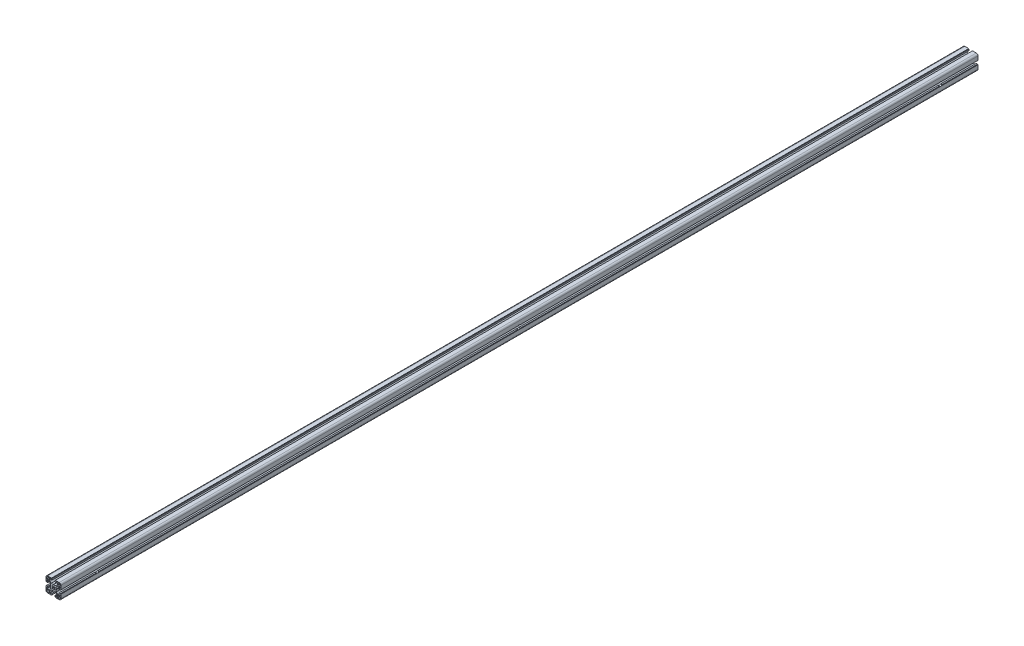
from build123d import *

# Parameters (mm, degrees)
EXTRUDE_1_DEPTH             = 2470
HOLE_WIZARD_2_D             = 6.6
HOLE_WIZARD_2_CBORE_D       = 11
HOLE_WIZARD_2_CBORE_DEPTH   = 6.8
HOLE_WIZARD_2_2_D           = 6.6
HOLE_WIZARD_2_2_CBORE_D     = 11
HOLE_WIZARD_2_2_CBORE_DEPTH = 6.8


with BuildPart() as part:
    # 草图1 → 凸台-拉伸1 (new body)
    with BuildSketch(Plane.XY):
        with BuildLine():
            Line((-18.9995, -4.100341675), (-18.9995, -5.100341675))
            Line((-18.9995, -5.100341675), (-19.9995, -5.100341675))
            Line((-19.9995, -5.100341675), (-19.9995, -15.500341675))
            ThreePointArc((-19.9995, -15.500341675), (-18.681480515, -18.682322191), (-15.4995, -20.000341675))
            Line((-15.4995, -20.000341675), (-5.0995, -20.000341675))
            Line((-5.0995, -20.000341675), (-5.0995, -19.000341675))
            Line((-5.0995, -19.000341675), (-4.0995, -19.000341675))
            Line((-4.0995, -19.000341675), (-4.0995, -15.500341675))
            Line((-4.0995, -15.500341675), (-6.5995, -15.500341675))
            Line((-6.5995, -15.500341675), (-6.5995, -16.500341675))
            ThreePointArc((-6.5995, -16.500341675), (-6.892393219, -17.207448457), (-7.5995, -17.500341675))
            Line((-7.5995, -17.500341675), (-9.7995, -17.500341675))
            ThreePointArc((-9.7995, -17.500341675), (-10.153053391, -17.353895066), (-10.2995, -17.000341675))
            Line((-10.2995, -17.000341675), (-10.2995, -11.997341675))
            Line((-10.2995, -11.997341675), (-5.9025, -7.600341675))
            Line((-5.9025, -7.600341675), (-0.5195, -7.600341675))
            Line((-0.5195, -7.600341675), (0.0005, -7.300341675))
            Line((0.0005, -7.300341675), (0.5195, -7.600341675))
            Line((0.5195, -7.600341675), (5.9035, -7.600341675))
            Line((5.9035, -7.600341675), (10.3005, -11.997341675))
            Line((10.3005, -11.997341675), (10.3005, -17.000341675))
            ThreePointArc((10.3005, -17.000341675), (10.154053391, -17.353895066), (9.8005, -17.500341675))
            Line((9.8005, -17.500341675), (7.6005, -17.500341675))
            ThreePointArc((7.6005, -17.500341675), (6.893393219, -17.207448457), (6.6005, -16.500341675))
            Line((6.6005, -16.500341675), (6.6005, -15.500341675))
            Line((6.6005, -15.500341675), (4.1005, -15.500341675))
            Line((4.1005, -15.500341675), (4.1005, -19.000341675))
            Line((4.1005, -19.000341675), (5.1005, -19.000341675))
            Line((5.1005, -19.000341675), (5.1005, -20.000341675))
            Line((5.1005, -20.000341675), (15.5005, -20.000341675))
            ThreePointArc((15.5005, -20.000341675), (18.682480515, -18.682322191), (20.0005, -15.500341675))
            Line((20.0005, -15.500341675), (20.0005, -5.100341675))
            Line((20.0005, -5.100341675), (19.0005, -5.100341675))
            Line((19.0005, -5.100341675), (19.0005, -4.100341675))
            Line((19.0005, -4.100341675), (15.5005, -4.100341675))
            Line((15.5005, -4.100341675), (15.5005, -6.600341675))
            Line((15.5005, -6.600341675), (16.5005, -6.600341675))
            ThreePointArc((16.5005, -6.600341675), (17.207606781, -6.893234894), (17.5005, -7.600341675))
            Line((17.5005, -7.600341675), (17.5005, -9.800341675))
            ThreePointArc((17.5005, -9.800341675), (17.354053391, -10.153895066), (17.0005, -10.300341675))
            Line((17.0005, -10.300341675), (11.9975, -10.300341675))
            Line((11.9975, -10.300341675), (7.6005, -5.903341675))
            Line((7.6005, -5.903341675), (7.6005, -0.520341675))
            Line((7.6005, -0.520341675), (7.3005, -0.000341675))
            Line((7.3005, -0.000341675), (7.6005, 0.519658325))
            Line((7.6005, 0.519658325), (7.6005, 5.902658325))
            Line((7.6005, 5.902658325), (11.9975, 10.299658325))
            Line((11.9975, 10.299658325), (17.0005, 10.299658325))
            ThreePointArc((17.0005, 10.299658325), (17.354053391, 10.153211715), (17.5005, 9.799658325))
            Line((17.5005, 9.799658325), (17.5005, 7.599658325))
            ThreePointArc((17.5005, 7.599658325), (17.207606781, 6.892551543), (16.5005, 6.599658325))
            Line((16.5005, 6.599658325), (15.5005, 6.599658325))
            Line((15.5005, 6.599658325), (15.5005, 4.099658325))
            Line((15.5005, 4.099658325), (19.0005, 4.099658325))
            Line((19.0005, 4.099658325), (19.0005, 5.099658325))
            Line((19.0005, 5.099658325), (20.0005, 5.099658325))
            Line((20.0005, 5.099658325), (20.0005, 15.499658325))
            ThreePointArc((20.0005, 15.499658325), (18.682480515, 18.68163884), (15.5005, 19.999658325))
            Line((15.5005, 19.999658325), (5.1005, 19.999658325))
            Line((5.1005, 19.999658325), (5.1005, 18.999658325))
            Line((5.1005, 18.999658325), (4.1005, 18.999658325))
            Line((4.1005, 18.999658325), (4.1005, 15.499658325))
            Line((4.1005, 15.499658325), (6.6005, 15.499658325))
            ThreePointArc((6.6005, 15.499658325), (6.393348977, 15.999658325), (6.6005, 16.499658325))
            ThreePointArc((6.6005, 16.499658325), (6.893393219, 17.206765106), (7.6005, 17.499658325))
            Line((7.6005, 17.499658325), (9.8005, 17.499658325))
            ThreePointArc((9.8005, 17.499658325), (10.154053391, 17.353211715), (10.3005, 16.999658325))
            Line((10.3005, 16.999658325), (10.3005, 11.996658325))
            Line((10.3005, 11.996658325), (5.9035, 7.599658325))
            Line((5.9035, 7.599658325), (0.5195, 7.599658325))
            Line((0.5195, 7.599658325), (0.0005, 7.299658325))
            Line((0.0005, 7.299658325), (-0.5195, 7.599658325))
            Line((-0.5195, 7.599658325), (-5.9025, 7.599658325))
            Line((-5.9025, 7.599658325), (-10.2995, 11.996658325))
            Line((-10.2995, 11.996658325), (-10.2995, 16.999658325))
            ThreePointArc((-10.2995, 16.999658325), (-10.153053391, 17.353211715), (-9.7995, 17.499658325))
            Line((-9.7995, 17.499658325), (-7.5995, 17.499658325))
            ThreePointArc((-7.5995, 17.499658325), (-6.892393219, 17.206765106), (-6.5995, 16.499658325))
            Line((-6.5995, 16.499658325), (-6.5995, 15.499658325))
            Line((-6.5995, 15.499658325), (-4.0995, 15.499658325))
            Line((-4.0995, 15.499658325), (-4.0995, 18.999658325))
            Line((-4.0995, 18.999658325), (-5.0995, 18.999658325))
            Line((-5.0995, 18.999658325), (-5.0995, 19.999658325))
            Line((-5.0995, 19.999658325), (-15.4995, 19.999658325))
            ThreePointArc((-15.4995, 19.999658325), (-18.681480515, 18.68163884), (-19.9995, 15.499658325))
            Line((-19.9995, 15.499658325), (-19.9995, 5.099658325))
            Line((-19.9995, 5.099658325), (-18.9995, 5.099658325))
            Line((-18.9995, 5.099658325), (-18.9995, 4.099658325))
            Line((-18.9995, 4.099658325), (-15.4995, 4.099658325))
            Line((-15.4995, 4.099658325), (-15.4995, 6.599658325))
            Line((-15.4995, 6.599658325), (-16.4995, 6.599658325))
            ThreePointArc((-16.4995, 6.599658325), (-17.206606781, 6.892551543), (-17.4995, 7.599658325))
            Line((-17.4995, 7.599658325), (-17.4995, 9.799658325))
            ThreePointArc((-17.4995, 9.799658325), (-17.353053391, 10.153211715), (-16.9995, 10.299658325))
            Line((-16.9995, 10.299658325), (-11.9965, 10.299658325))
            Line((-11.9965, 10.299658325), (-7.5995, 5.902658325))
            Line((-7.5995, 5.902658325), (-7.5995, 0.519658325))
            Line((-7.5995, 0.519658325), (-7.2995, -0.000341675))
            Line((-7.2995, -0.000341675), (-7.5995, -0.520341675))
            Line((-7.5995, -0.520341675), (-7.5995, -5.903341675))
            Line((-7.5995, -5.903341675), (-11.9965, -10.300341675))
            Line((-11.9965, -10.300341675), (-16.9995, -10.300341675))
            ThreePointArc((-16.9995, -10.300341675), (-17.353053391, -10.153895066), (-17.4995, -9.800341675))
            Line((-17.4995, -9.800341675), (-17.4995, -7.600341675))
            ThreePointArc((-17.4995, -7.600341675), (-17.206606781, -6.893234894), (-16.4995, -6.600341675))
            Line((-16.4995, -6.600341675), (-15.4995, -6.600341675))
            Line((-15.4995, -6.600341675), (-15.4995, -4.100341675))
            Line((-15.4995, -4.100341675), (-18.9995, -4.100341675))
        make_face()
        with BuildLine():
            Line((15.5005, -18.000341675), (11.8005, -18.000341675))
            Line((11.8005, -18.000341675), (11.8005, -11.800341675))
            Line((11.8005, -11.800341675), (18.0005, -11.800341675))
            Line((18.0005, -11.800341675), (18.0005, -15.500341675))
            ThreePointArc((18.0005, -15.500341675), (17.268266953, -17.268108628), (15.5005, -18.000341675))
        make_face(mode=Mode.SUBTRACT)
        with BuildLine():
            Line((18.0005, 11.799658325), (11.8005, 11.799658325))
            Line((11.8005, 11.799658325), (11.8005, 17.999658325))
            Line((11.8005, 17.999658325), (15.5005, 17.999658325))
            ThreePointArc((15.5005, 17.999658325), (17.268266953, 17.267425278), (18.0005, 15.499658325))
            Line((18.0005, 15.499658325), (18.0005, 11.799658325))
        make_face(mode=Mode.SUBTRACT)
        with BuildLine():
            Line((-1.8145, -2.875341675), (-3.004391671, -4.066450004))
            Line((-3.004391671, -4.066450004), (-4.065608329, -3.005233346))
            Line((-4.065608329, -3.005233346), (-2.8745, -1.815341675))
            ThreePointArc((-2.8745, -1.815341675), (-3.399473913, -0.000341675), (-2.8745, 1.814658325))
            Line((-2.8745, 1.814658325), (-4.064391671, 3.005766654))
            Line((-4.064391671, 3.005766654), (-3.004391671, 4.065766654))
            Line((-3.004391671, 4.065766654), (-1.8145, 2.874658325))
            ThreePointArc((-1.8145, 2.874658325), (0, 3.399316649), (1.8145, 2.874658325))
            Line((1.8145, 2.874658325), (3.0055, 4.065658325))
            Line((3.0055, 4.065658325), (4.066608329, 3.004549996))
            Line((4.066608329, 3.004549996), (2.8755, 1.814658325))
            ThreePointArc((2.8755, 1.814658325), (3.400473913, -0.000341675), (2.8755, -1.815341675))
            Line((2.8755, -1.815341675), (4.066608329, -3.005233346))
            Line((4.066608329, -3.005233346), (3.0055, -4.066341675))
            Line((3.0055, -4.066341675), (1.8145, -2.875341675))
            ThreePointArc((1.8145, -2.875341675), (0, -3.4), (-1.8145, -2.875341675))
        make_face(mode=Mode.SUBTRACT)
        with BuildLine():
            Line((-17.9995, -15.500341675), (-17.9995, -11.800341675))
            Line((-17.9995, -11.800341675), (-11.7995, -11.800341675))
            Line((-11.7995, -11.800341675), (-11.7995, -18.000341675))
            Line((-11.7995, -18.000341675), (-15.4995, -18.000341675))
            ThreePointArc((-15.4995, -18.000341675), (-17.267266953, -17.268108628), (-17.9995, -15.500341675))
        make_face(mode=Mode.SUBTRACT)
        with BuildLine():
            Line((-11.7995, 17.999658325), (-11.7995, 11.799658325))
            Line((-11.7995, 11.799658325), (-17.9995, 11.799658325))
            Line((-17.9995, 11.799658325), (-17.9995, 15.499658325))
            ThreePointArc((-17.9995, 15.499658325), (-17.267266953, 17.267425278), (-15.4995, 17.999658325))
            Line((-15.4995, 17.999658325), (-11.7995, 17.999658325))
        make_face(mode=Mode.SUBTRACT)
    extrude(amount=-EXTRUDE_1_DEPTH)

    # Hole Wizard 2 (through all)
    with Locations(Plane(origin=(20.0005, 0, 0), x_dir=(0, 0, -1), z_dir=(1, 0, 0))):
        with Locations((2370, -0.000341675), (1235, 0.519658325), (99.999999999, -0.000341675)):
            CounterBoreHole(HOLE_WIZARD_2_D / 2, HOLE_WIZARD_2_CBORE_D / 2, HOLE_WIZARD_2_CBORE_DEPTH)

    # Hole Wizard 2 2 (through all)
    with Locations(Plane.ZY.offset(19.9995)):
        with Locations((-99.999999999, -0.000341675), (-1235, 0.519658325), (-2370, -0.000341675)):
            CounterBoreHole(HOLE_WIZARD_2_2_D / 2, HOLE_WIZARD_2_2_CBORE_D / 2, HOLE_WIZARD_2_2_CBORE_DEPTH)


solid = part.part
